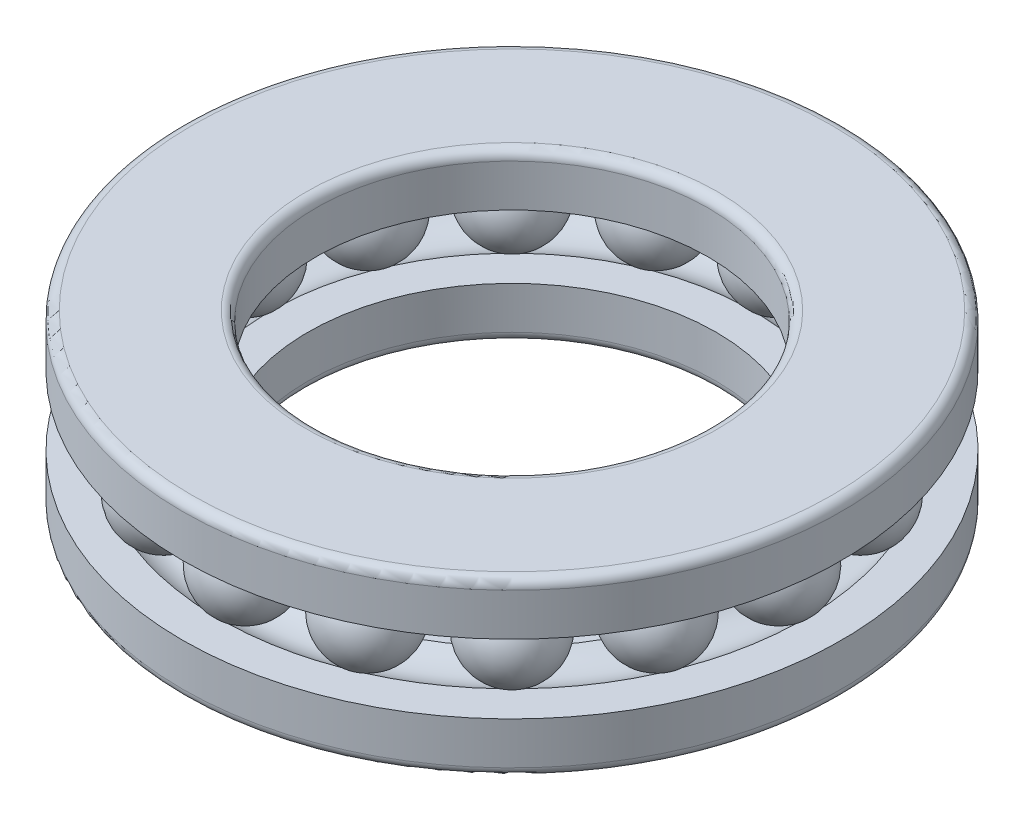
from build123d import *

# Parameters (mm, degrees)
CIRPATTERN1_COUNT = 16
FILLET1_R         = 0.6


with BuildPart() as part:
    # Sketch2 → Base-Revolve (revolve)
    with BuildSketch(Plane.XY, mode=Mode.PRIVATE) as base_revolve_sk:
        with BuildLine():
            Line((0, 3.3), (2.35, 3.3))
            ThreePointArc((2.35, 3.3), (4, 2.75), (5.65, 3.3))
            Line((5.65, 3.3), (8, 3.3))
            Line((8, 3.3), (8, 0))
            Line((8, 0), (0, 0))
            Line((0, 0), (0, 3.3))
        make_face()
    revolve(base_revolve_sk.sketch.rotate(Axis((21, 0, 0), (0, 1, 0)), 270), axis=Axis((21, 0, 0), (0, 1, 0)))

    # Sketch3 → Boss-Revolve2 (revolve)
    with BuildSketch(Plane.XY):
        with BuildLine():
            Line((4, 2.7), (4, 8.3))
            ThreePointArc((4, 8.3), (1.2, 5.5), (4, 2.7))
        make_face()
    boss_revolve2 = revolve(axis=Axis((4, 0, 0), (0, 1, 0)))

    # Sketch4 → Boss-Revolve3 (revolve)
    with BuildSketch(Plane.XY, mode=Mode.PRIVATE) as boss_revolve3_sk:
        with BuildLine():
            Line((0, 7.7), (2.35, 7.7))
            ThreePointArc((2.35, 7.7), (4, 8.25), (5.65, 7.7))
            Line((5.65, 7.7), (8.5, 7.7))
            Line((8.5, 7.7), (8.5, 11))
            Line((8.5, 11), (0, 11))
            Line((0, 11), (0, 7.7))
        make_face()
    revolve(boss_revolve3_sk.sketch.rotate(Axis((21, 0, 0), (0, 1, 0)), 270), axis=Axis((21, 0, 0), (0, 1, 0)))

    # CirPattern1: Boss-Revolve2 ×16 about axis
    cirpattern1_axis = Axis((21, 0, 0), (0, 1, 0))
    for i in range(1, CIRPATTERN1_COUNT):
        add(boss_revolve2.rotate(cirpattern1_axis, i * 360 / CIRPATTERN1_COUNT))

    # Fillet1
    fillet1_edges = [part.edges().sort_by_distance(p)[0] for p in [
        (21, 11, 12.5),
        (21, 11, 21),
        (21, 0, 13),
        (21, 0, 21),
    ]]
    fillet(fillet1_edges, radius=FILLET1_R)


solid = part.part
